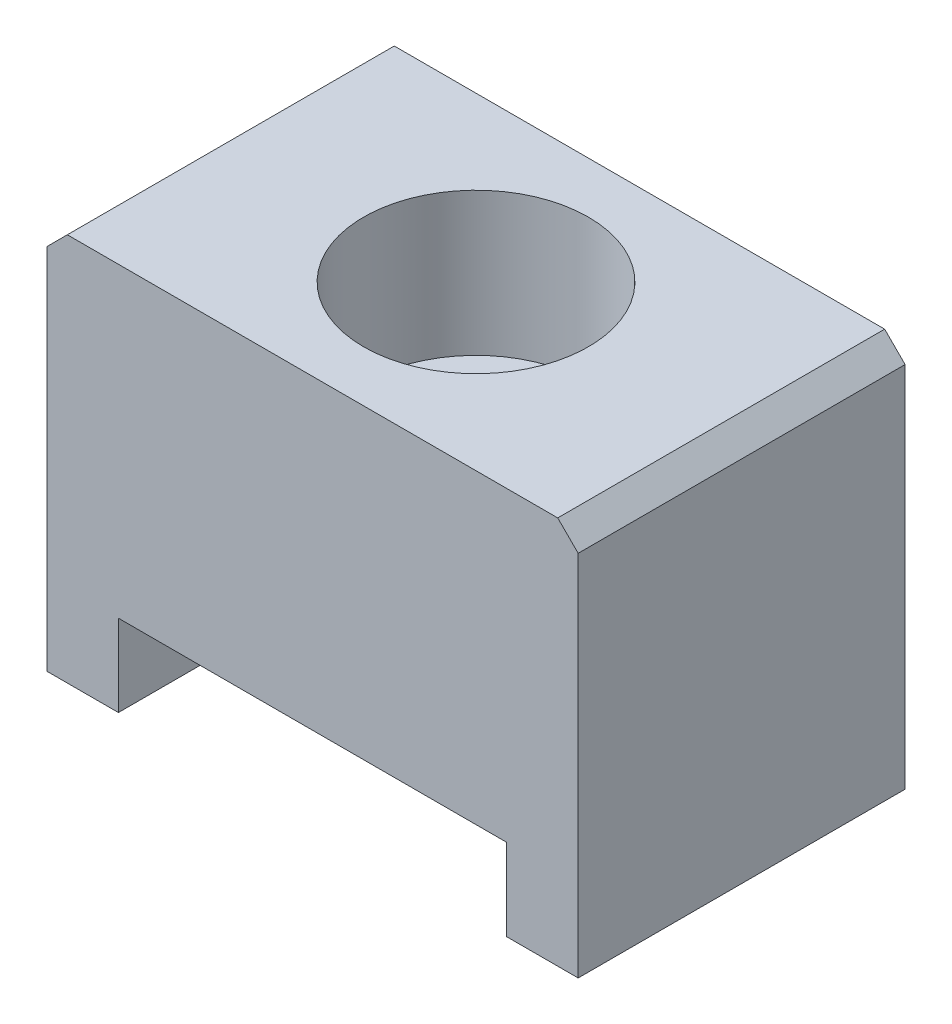
from build123d import *

# Parameters (mm, degrees)
BOSS_EXTRUDE1_DEPTH = 16
SKETCH2_R           = 5.5
CUT_EXTRUDE1_DEPTH  = 7
SKETCH3_R           = 3.5
CUT_EXTRUDE2_DEPTH  = 8
CHAMFER1_SIZE       = 1


with BuildPart() as part:
    # Sketch1 → Boss-Extrude1 (new body)
    with BuildSketch(Plane.XY):
        Polygon((0, 0), (0, 19), (26, 19), (26, 0), (22.5, 0), (22.5, 4), (3.5, 4), (3.5, 0), align=None)
    extrude(amount=BOSS_EXTRUDE1_DEPTH)

    # Sketch2 → Cut-Extrude1 (cut)
    with BuildSketch(Plane(origin=(0, 19, 0), x_dir=(1, 0, 0), z_dir=(0, 1, 0))):
        with Locations(Location((13, -8, 0), (0, 0, 270))):
            Circle(SKETCH2_R)
    extrude(amount=-CUT_EXTRUDE1_DEPTH, mode=Mode.SUBTRACT)

    # Sketch3 → Cut-Extrude2 (cut)
    with BuildSketch(Plane(origin=(0, 12, 0), x_dir=(1, 0, 0), z_dir=(0, 1, 0))):
        with Locations(Location((13, -8, 0), (0, 0, 270))):
            Circle(SKETCH3_R)
    extrude(amount=-CUT_EXTRUDE2_DEPTH, mode=Mode.SUBTRACT)

    # Chamfer1
    chamfer1_edges = [part.edges().sort_by_distance(p)[0] for p in [
        (0, 19, 8),
        (26, 19, 8),
    ]]
    chamfer(chamfer1_edges, length=CHAMFER1_SIZE)


solid = part.part
